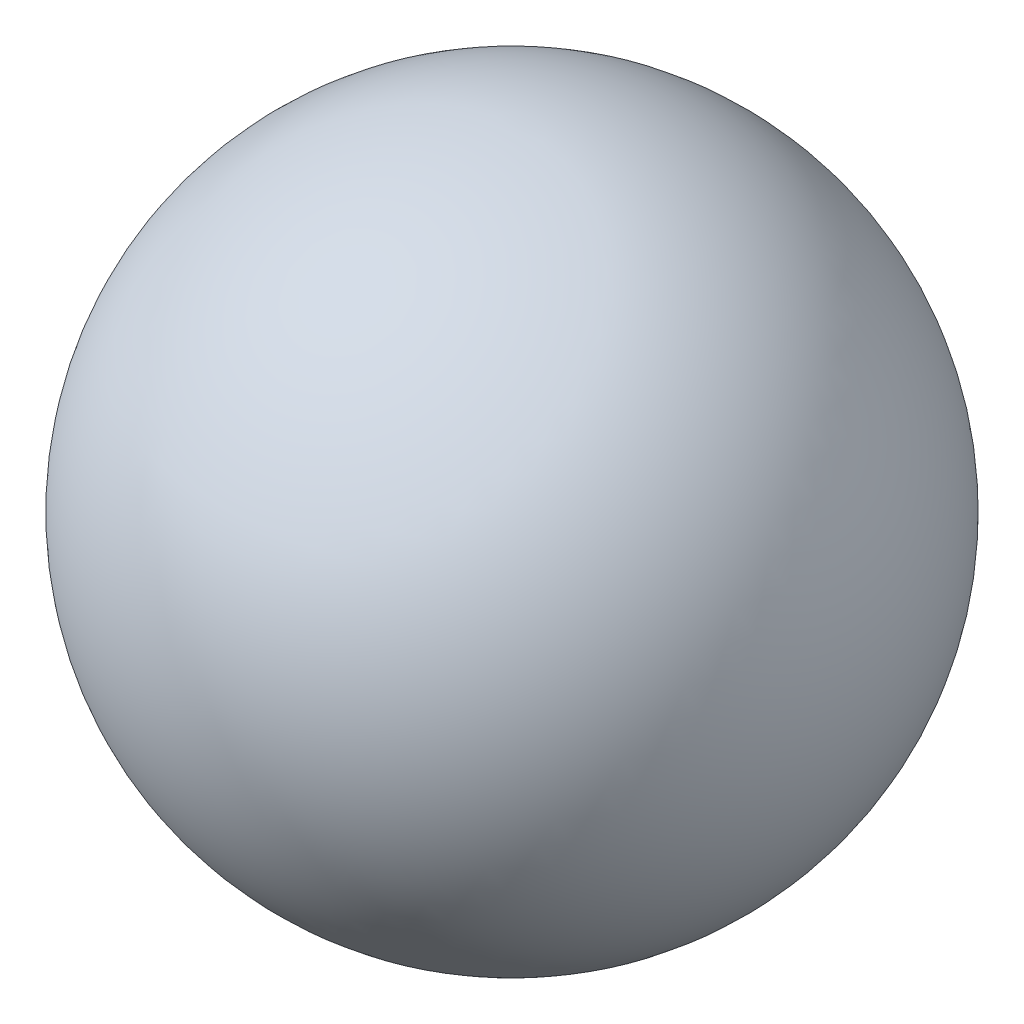
from build123d import *


with BuildPart() as part:
    # Sketch1 → Revolve1 (revolve)
    with BuildSketch(Plane.XY):
        with BuildLine():
            Line((0, 0), (0, 5.5))
            ThreePointArc((0, 5.5), (-2.75, 2.75), (0, 0))
        make_face()
    revolve(axis=Axis((0, 0, 0), (0, 1, 0)))


solid = part.part
